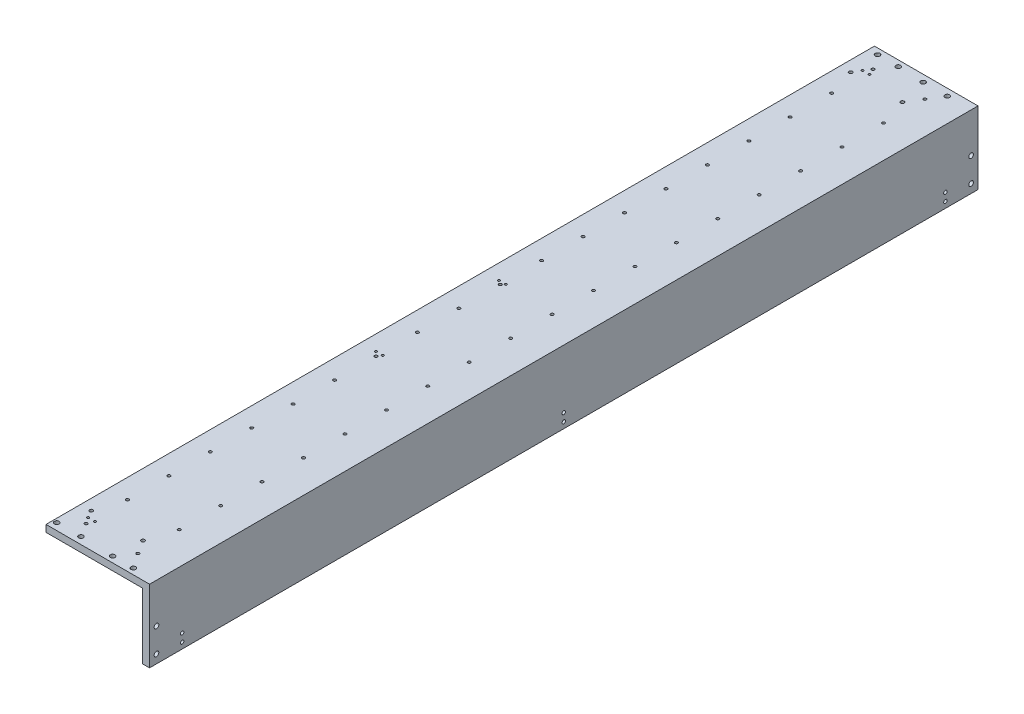
from build123d import *

# Parameters (mm, degrees)
EXTRUDE_1_DEPTH    = 600
HOLE_WIZARD_M8_1_D = 6.8
HOLE_WIZARD_M8_2_D = 6.8
HOLE_WIZARD_M5_1_D = 4.2
F_5_0MM_1_D        = 5
HOLE_WIZARD_M4_1_D = 3.3
HOLE_WIZARD_M6_1_D = 5
MOVE_FACE_1_BY     = 10
HOLE_WIZARD_M8_3_D = 6.8


with BuildPart() as part:
    # 草图1 → 凸台-拉伸1 (new, symmetric)
    with BuildSketch(Plane.XY):
        Polygon((0, 0), (160, 0), (160, -105), (150, -105), (150, -10), (0, -10), align=None)
    extrude(amount=EXTRUDE_1_DEPTH, both=True)

    # M8 螺纹孔1 (through all)
    with Locations(Plane(origin=(0, 0, 0), x_dir=(1, 0, 0), z_dir=(0, 1, 0))):
        with Locations((15.5, -590), (50.5, -590), (90.5, 590), (125.5, 590)):
            Hole(HOLE_WIZARD_M8_1_D / 2)

    # M8 螺纹孔2 (through all)
    with Locations(Plane(origin=(160, 0, 0), x_dir=(0, 0, -1), z_dir=(1, 0, 0))):
        with Locations((-590, -57.5), (-590, -92.5), (590, -92.5), (590, -57.5)):
            Hole(HOLE_WIZARD_M8_2_D / 2)

    # M5 螺纹孔1 (through all)
    with Locations(Plane(origin=(0, -10, 0), x_dir=(-1, 0, 0), z_dir=(0, -1, 0))):
        with Locations((-38, -570), (-38, -510), (-38, -450), (-38, -390), (-38, -330), (-38, -270), (-38, -210), (-38, -150), (-38, -90), (-38, -30), (-38, 30), (-38, 90), (-38, 150), (-38, 210), (-38, 270), (-38, 330), (-38, 390), (-38, 450), (-38, 510), (-38, 570), (-113, -570), (-113, -510), (-113, -450), (-113, -390), (-113, -330), (-113, -270), (-113, -210), (-113, -150), (-113, -90), (-113, -30), (-113, 30), (-113, 90), (-113, 150), (-113, 210), (-113, 270), (-113, 330), (-113, 390), (-113, 450), (-113, 510), (-113, 570)):
            Hole(HOLE_WIZARD_M5_1_D / 2)

    # Ø5.0mm 暗销孔1 (through all)
    with Locations(Plane(origin=(0, -10, 0), x_dir=(-1, 0, 0), z_dir=(0, -1, 0))):
        with Locations((-25.5, 550), (-25.5, -550), (-100.5, 550), (-100.5, -550)):
            Hole(F_5_0MM_1_D / 2)

    # M4 螺纹孔1 (through all)
    with Locations(Plane(origin=(0, 0, 0), x_dir=(1, 0, 0), z_dir=(0, 1, 0))):
        with Locations((31.978248954, 560.9), (41.878248954, 560.9), (31.978248954, 34.1), (41.878248954, 34.1), (31.978248954, -144.1), (41.878248954, -144.1), (31.978248954, -560.9), (41.878248954, -560.9)):
            Hole(HOLE_WIZARD_M4_1_D / 2)

    # M6 螺纹孔1 (through all)
    with Locations(Plane(origin=(160, 0, 0), x_dir=(0, 0, -1), z_dir=(1, 0, 0))):
        with Locations((-552.8, -84.790968568), (-552.8, -96.290968568), (0, -84.790968568), (0, -96.290968568), (552.8, -84.790968568), (552.8, -96.290968568)):
            Hole(HOLE_WIZARD_M6_1_D / 2)

    # Move Face 1: a face moved inward by 10.0
    extrude(part.faces().sort_by_distance((0, -5, 0))[0], amount=MOVE_FACE_1_BY, dir=(1, 0, 0), mode=Mode.SUBTRACT)

    # M8 螺纹孔3 (through all)
    with Locations(Plane(origin=(0, -10, 0), x_dir=(-1, 0, 0), z_dir=(0, -1, 0))):
        with Locations((-53, 591.5), (-23, 591.5), (-128.000000121, -591.5), (-97.999999879, -591.5)):
            Hole(HOLE_WIZARD_M8_3_D / 2)


solid = part.part
